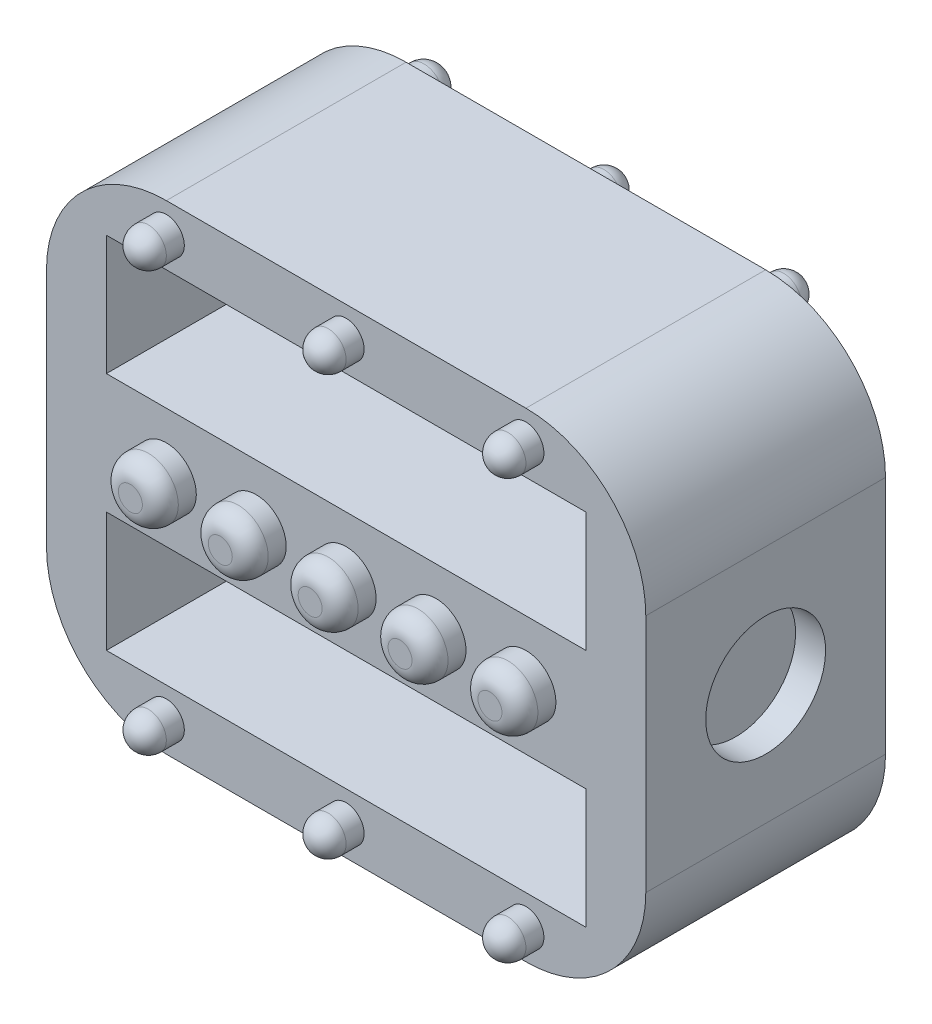
from build123d import *

# Parameters (mm, degrees)
SKETCH1_W           = 10
SKETCH1_H           = 8
SKETCH1_W_2         = 8
SKETCH1_H_2         = 2
BOSS_EXTRUDE3_DEPTH = 4
SKETCH2_R           = 1
CUT_EXTRUDE6_DEPTH  = 0.5
FILLET1_R           = 2
SKETCH4_R           = 0.5
SKETCH4_R_2         = 0.3
BOSS_EXTRUDE7_DEPTH = 0.6
FILLET4_R           = 0.3
BOSS_EXTRUDE8_START = 0.6
SKETCH5_R           = 0.5
SKETCH5_R_2         = 0.3
SKETCH5_R_3         = 0.325
BOSS_EXTRUDE8_DEPTH = 0.6
FILLET5_R           = 0.3
FILLET6_R           = 0.3
FILLET7_R           = 0.3


with BuildPart() as part:
    # Sketch1 → Boss-Extrude3 (new body)
    with BuildSketch(Plane.XY):
        Rectangle(SKETCH1_W, SKETCH1_H)
        with Locations((0, 2)):
            Rectangle(SKETCH1_W_2, SKETCH1_H_2, mode=Mode.SUBTRACT)
        with Locations((0, -2)):
            Rectangle(SKETCH1_W_2, SKETCH1_H_2, mode=Mode.SUBTRACT)
    extrude(amount=BOSS_EXTRUDE3_DEPTH)

    # Sketch2 → Cut-Extrude6 (cut)
    with BuildSketch(Plane(origin=(5, 0, 0), x_dir=(0, 0, -1), z_dir=(1, 0, 0))):
        with Locations(Location((-2, 0, 0), (0, 0, 90))):
            Circle(SKETCH2_R)
    extrude(amount=-CUT_EXTRUDE6_DEPTH, mode=Mode.SUBTRACT)

    # Fillet1
    fillet1_edges = [part.edges().sort_by_distance(p)[0] for p in [
        (5, -4, 2),
        (-5, -4, 2),
        (-5, 4, 2),
        (5, 4, 2),
    ]]
    fillet(fillet1_edges, radius=FILLET1_R)

    # Sketch4 → Boss-Extrude7 (add)
    with BuildSketch(Plane.XY.offset(4)):
        Circle(SKETCH4_R)
        with Locations((-1.5, 0)):
            Circle(SKETCH4_R)
        with Locations((-3, 0)):
            Circle(SKETCH4_R)
        with Locations((1.5, 0)):
            Circle(SKETCH4_R)
        with Locations((3, 0)):
            Circle(SKETCH4_R)
        with Locations((3, -3.5)):
            Circle(SKETCH4_R_2)
        with Locations((0, -3.5)):
            Circle(SKETCH4_R_2)
        with Locations((-3, -3.5)):
            Circle(SKETCH4_R_2)
        with Locations((3, 3.5)):
            Circle(SKETCH4_R_2)
        with Locations((0, 3.5)):
            Circle(SKETCH4_R_2)
        with Locations((-3, 3.5)):
            Circle(SKETCH4_R_2)
    extrude(amount=BOSS_EXTRUDE7_DEPTH)

    # Fillet4
    fillet4_edges = [part.edges().sort_by_distance(p)[0] for p in [
        (-0.5, 0, 4.6),
        (-2, 0, 4.6),
        (-3.5, 0, 4.6),
        (1, 0, 4.6),
        (2.5, 0, 4.6),
    ]]
    fillet(fillet4_edges, radius=FILLET4_R)

    # Sketch5 → Boss-Extrude8 (add)
    with BuildSketch(Plane(origin=(0, 0, 0), x_dir=(-1, 0, 0), z_dir=(0, 0, -1)).offset(BOSS_EXTRUDE8_START)):
        with Locations(Location((0, 0, 0), (0, 0, 180))):
            Circle(SKETCH5_R)
        with Locations(Location((1.5, 0, 0), (0, 0, 180))):
            Circle(SKETCH5_R)
        with Locations(Location((3, 0, 0), (0, 0, 180))):
            Circle(SKETCH5_R)
        with Locations(Location((-1.5, 0, 0), (0, 0, 180))):
            Circle(SKETCH5_R)
        with Locations(Location((-3, 0, 0), (0, 0, 180))):
            Circle(SKETCH5_R)
        with Locations(Location((-3, 3.5, 0), (0, 0, 180))):
            Circle(SKETCH5_R_2)
        with Locations(Location((0, 3.5, 0), (0, 0, 180))):
            Circle(SKETCH5_R_2)
        with Locations(Location((3, 3.5, 0), (0, 0, 180))):
            Circle(SKETCH5_R_3)
        with Locations(Location((-3, -3.5, 0), (0, 0, 180))):
            Circle(SKETCH5_R_2)
        with Locations(Location((0, -3.5, 0), (0, 0, 180))):
            Circle(SKETCH5_R_2)
        with Locations(Location((3, -3.5, 0), (0, 0, 180))):
            Circle(SKETCH5_R_2)
    extrude(amount=-BOSS_EXTRUDE8_DEPTH)

    # Fillet5
    fillet5_edges = [part.edges().sort_by_distance(p)[0] for p in [
        (-0.5, 0, -0.6),
        (-2, 0, -0.6),
        (-3.5, 0, -0.6),
        (1, 0, -0.6),
        (2.5, 0, -0.6),
    ]]
    fillet(fillet5_edges, radius=FILLET5_R)

    # Fillet6
    fillet6_edges = [part.edges().sort_by_distance(p)[0] for p in [
        (-0.3, 3.5, 4.6),
        (-3.3, 3.5, 4.6),
        (2.7, -3.5, 4.6),
        (-0.3, -3.5, 4.6),
        (-3.3, -3.5, 4.6),
        (2.7, 3.5, 4.6),
    ]]
    fillet(fillet6_edges, radius=FILLET6_R)

    # Fillet7
    fillet7_edges = [part.edges().sort_by_distance(p)[0] for p in [
        (2.7, 3.5, -0.6),
        (-0.3, 3.5, -0.6),
        (-3.325, 3.5, -0.6),
        (2.7, -3.5, -0.6),
        (-0.3, -3.5, -0.6),
        (-3.3, -3.5, -0.6),
    ]]
    fillet(fillet7_edges, radius=FILLET7_R)


solid = part.part
